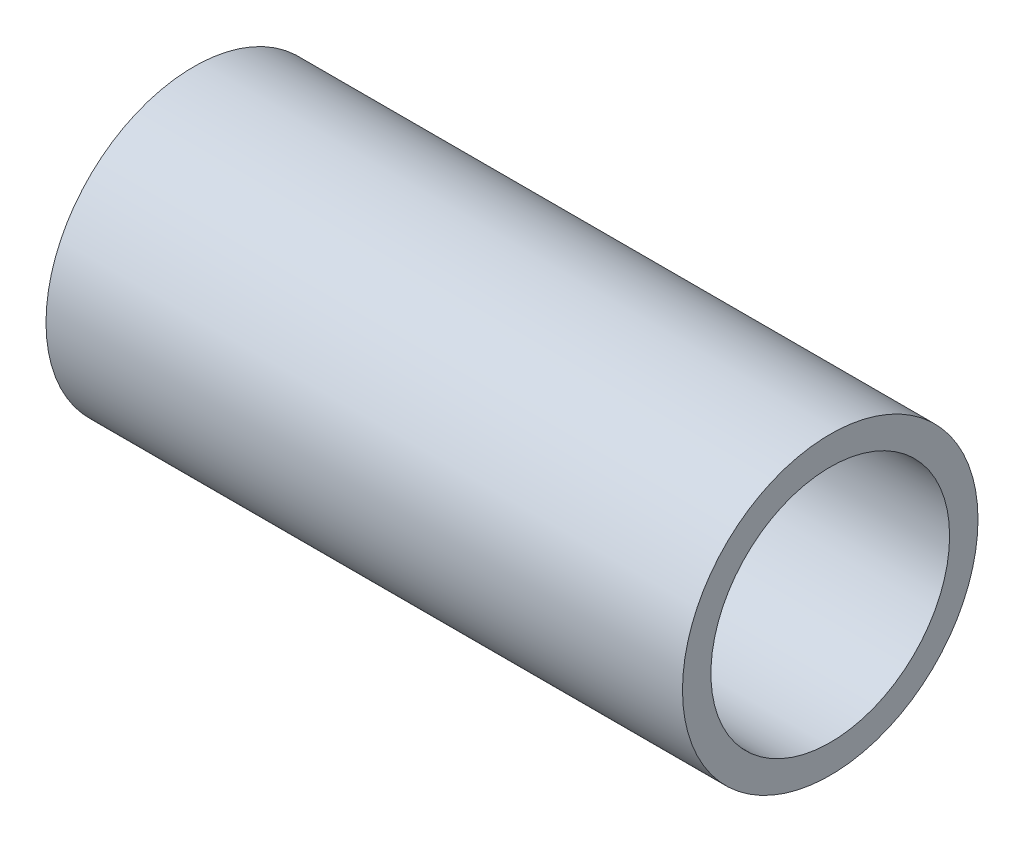
SolidWorks part; units mm, degrees
material "Q235"
ref_plane "Front Plane" through (0, 0, 0) normal (0, 0, 1) x (1, 0, 0)
ref_plane "Top Plane" through (0, 0, 0) normal (0, 1, 0) x (1, 0, 0)
ref_plane "Right Plane" through (0, 0, 0) normal (1, 0, 0) x (0, 0, -1)
sketch "Sketch1" plane through (0, 0, 0) normal (1, 0, 0) x (0, 0, -1)
  circle A0 centre (0, 0) radius 10.5
  circle A1 centre (0, 0) radius 13
  dimension "D1" = 21
  dimension "D2" = 26
extrude "Boss-Extrude1" add sketch "Sketch1" along normal blind 56
